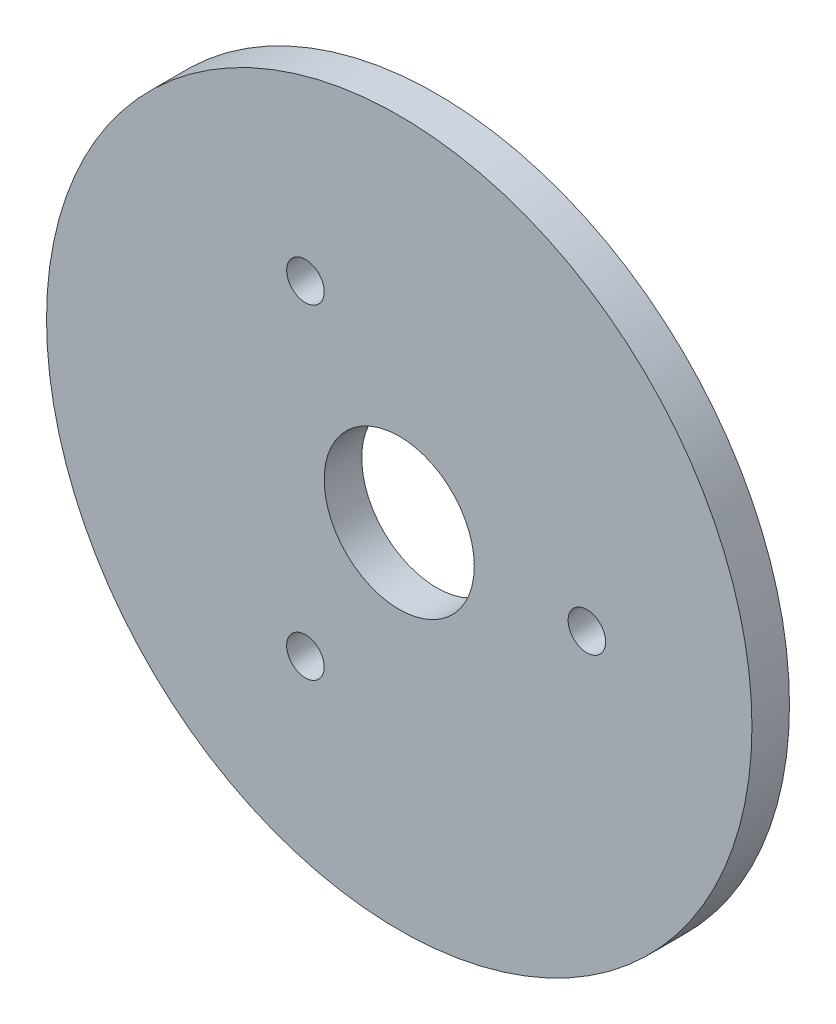
SolidWorks part; units mm, degrees
ref_plane "Front Plane" through (0, 0, 0) normal (0, 0, 1) x (1, 0, 0)
ref_plane "Top Plane" through (0, 0, 0) normal (0, 1, 0) x (1, 0, 0)
ref_plane "Right Plane" through (0, 0, 0) normal (1, 0, 0) x (0, 0, -1)
sketch "Sketch1" plane through (0, 0, 0) normal (0, 0, 1) x (1, 0, 0)
  circle A0 centre (0, 0) radius 10
  circle A1 centre (0, 0) radius 47
  circle A2 centre (0, 0) radius 25 construction
  circle A3 centre (25, 0) radius 2.5
  circle A4 centre (-12.5, -21.6506) radius 2.5
  circle A5 centre (-12.5, 21.6506) radius 2.5
  point P14 (0, 0)
  dimension "D1" = 94
  dimension "D2" = 20
  dimension "D3" = 50
  dimension "D4" = 5
  dimension "D5" = 3
extrude "Boss-Extrude1" add sketch "Sketch1" along normal blind 5
